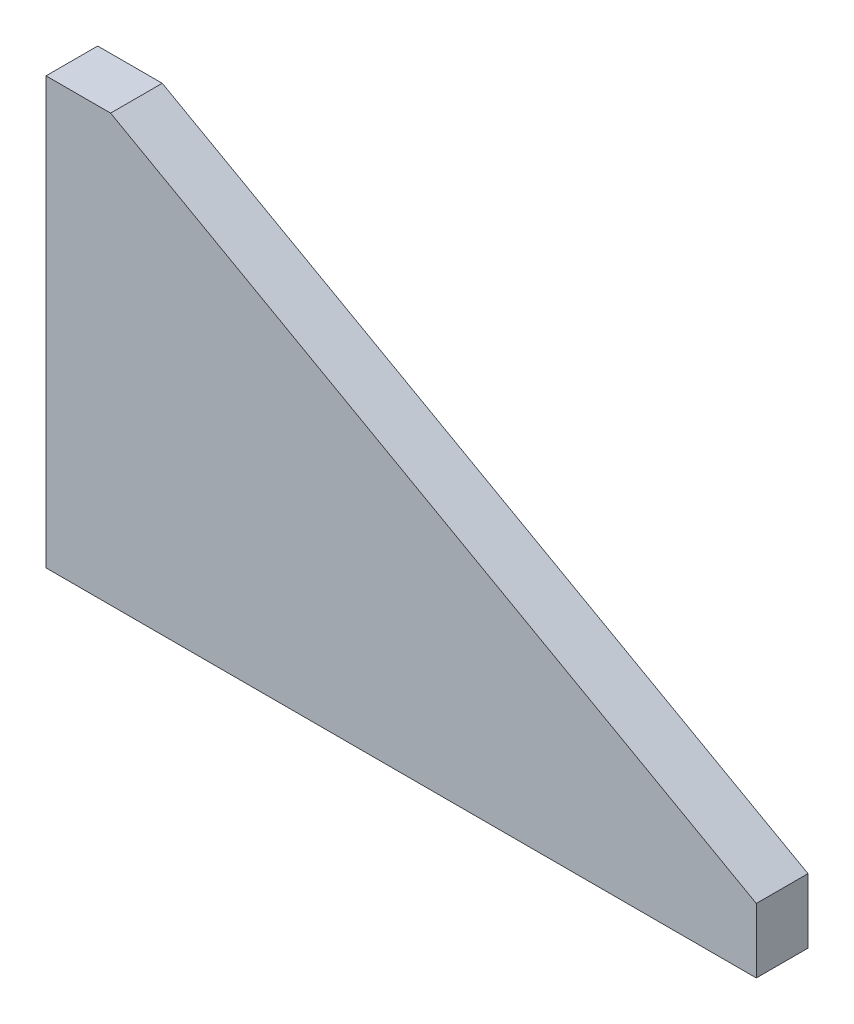
SolidWorks part; units mm, degrees
material "Q235B"
ref_plane "Front Plane" through (0, 0, 0) normal (0, 0, 1) x (1, 0, 0)
ref_plane "Top Plane" through (0, 0, 0) normal (0, 1, 0) x (1, 0, 0)
ref_plane "Right Plane" through (0, 0, 0) normal (1, 0, 0) x (0, 0, -1)
sketch "Sketch1" plane through (0, 0, 0) normal (0, 0, 1) x (1, 0, 0)
  line L0 (10, 66) -> (110, 10)
  line L1 (0, 0) -> (110, 0)
  line L2 (0, 0) -> (0, 66)
  line L3 (0, 66) -> (10, 66)
  line L4 (110, 0) -> (110, 10)
  point P7 (110, 66)
  point P9 (110, 66)
  dimension "D3" = 10
  dimension "D1" = 66
  dimension "D2" = 110
  dimension "D4" = 10
extrude "Boss-Extrude1" add sketch "Sketch1" along normal blind 8
